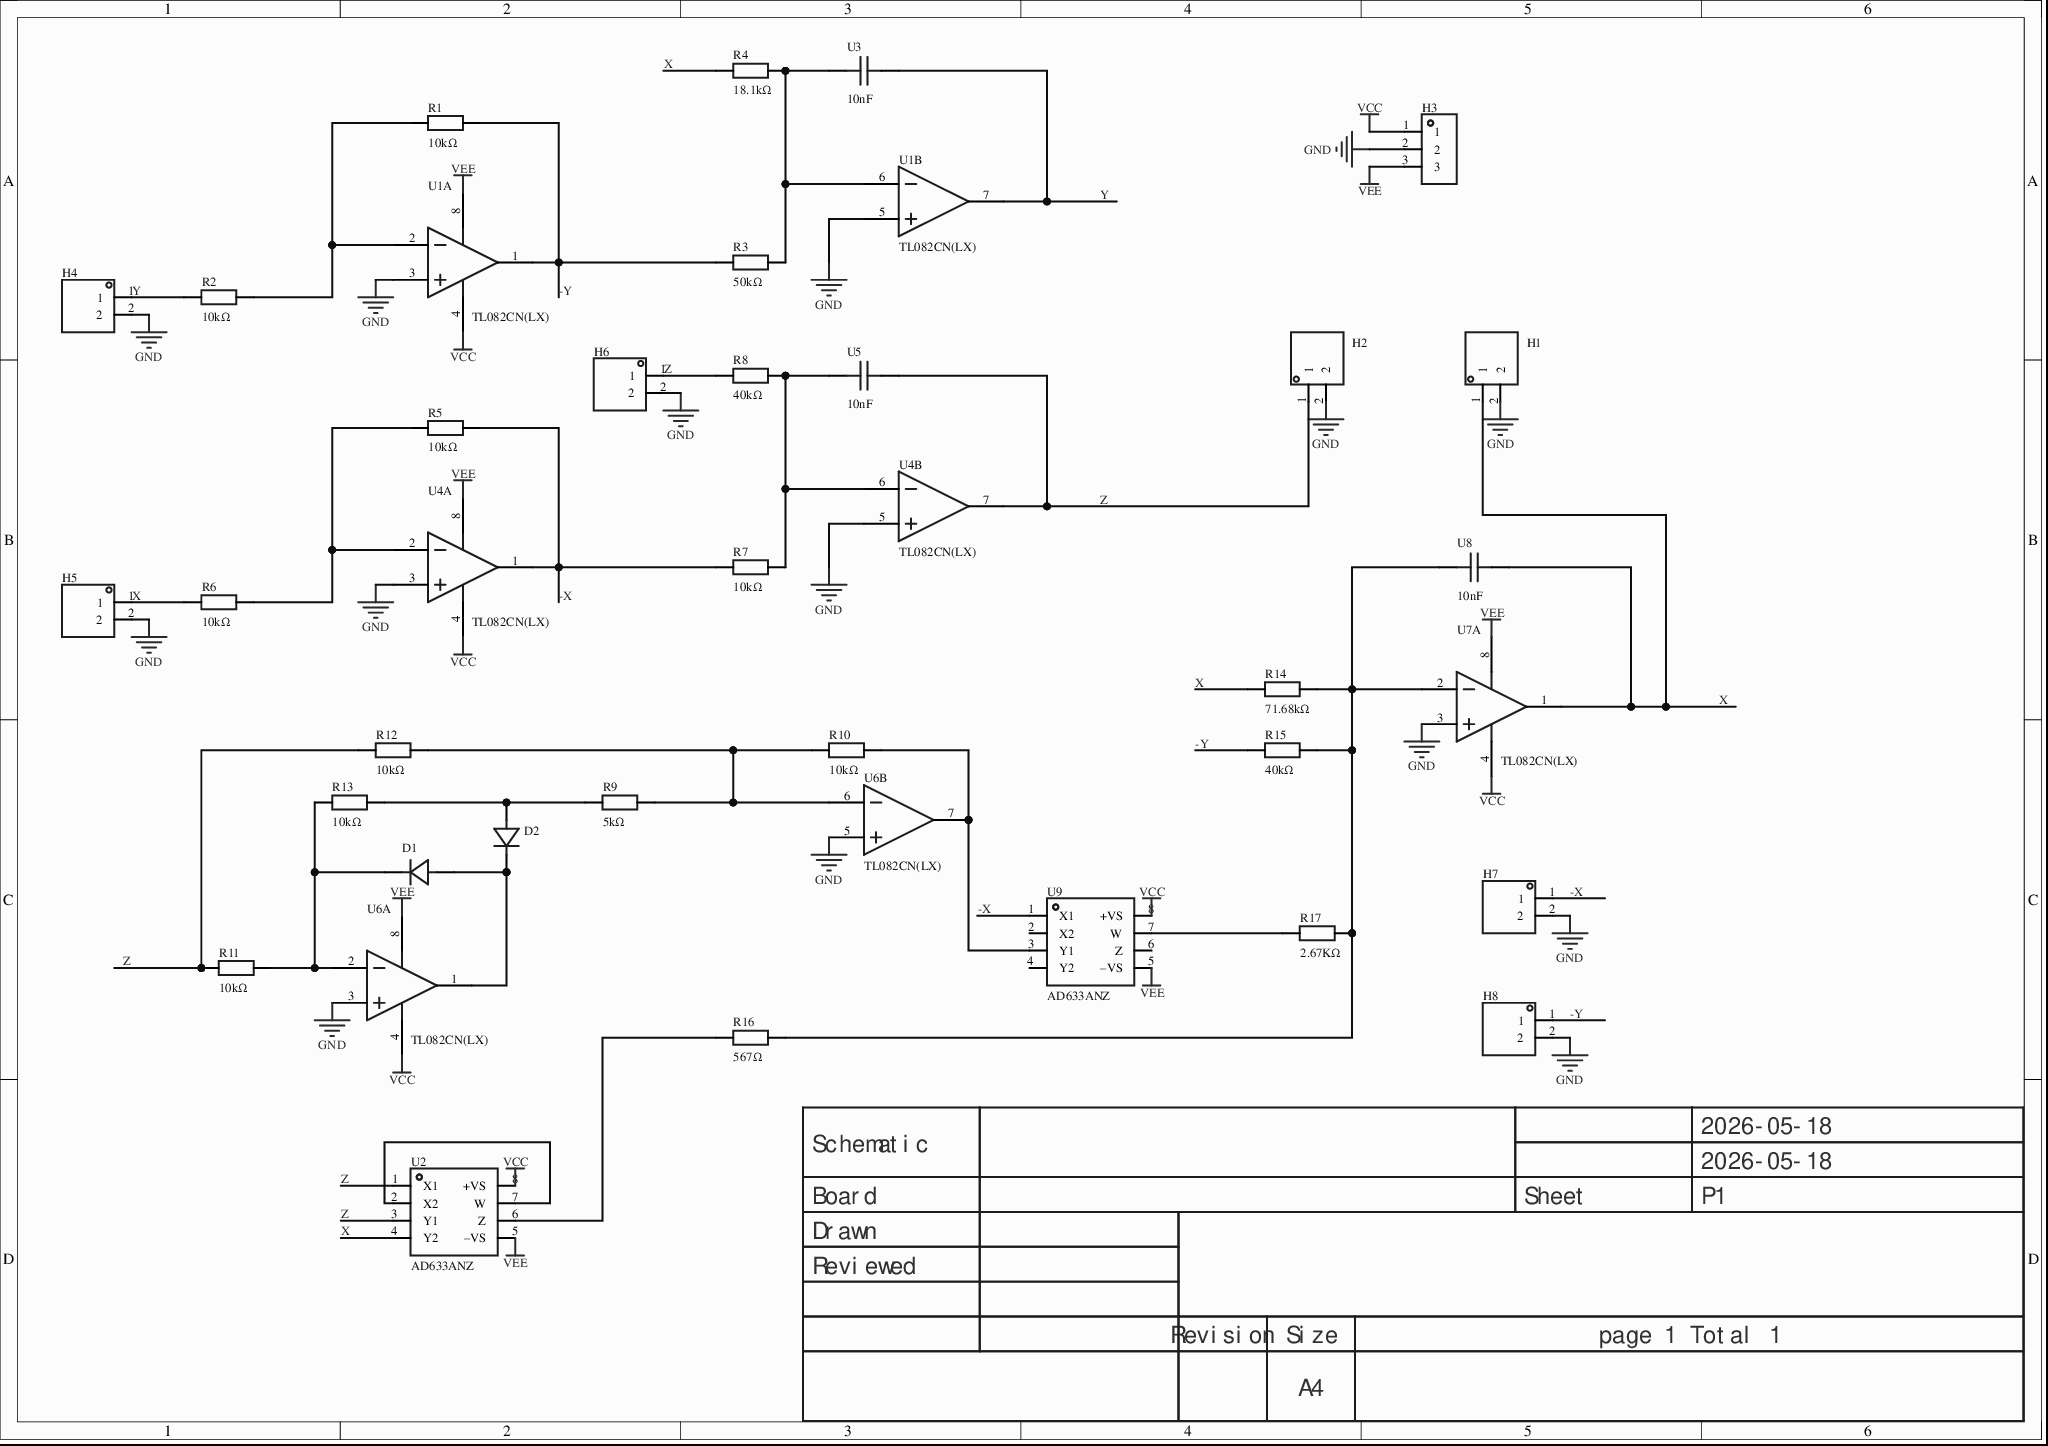
[diagram p0: MISC51419-3.schdoc]
# Altium project MISC51419-2.PrjPcb
1 sheet, 36 parts. Net scope: global (net labels, ports and power ports of the same name join across sheets).
Board file: MISC51419.pcbdoc

## Sheet MISC51419-3.schdoc
size 297 x 209 mm; Version: V1.0; @Project Name: MISC51419; @Update Date: 2026-05-18; @Create Date: 2026-05-18; @Board Name: MISC51419; @Create Time: 16:48:40; @Page Count: 1; @Page No: 1; @Schematic Name: MISC51419; @Update Time: 16:48:40; Size: A4

### Parts
D1  (no value)  [DO_1N4007]
D2  (no value)  [DO_1N4007]
H1  (no value)  [HDR-TH_2P-P2.54-V-M-1]
H2  (no value)  [HDR-TH_2P-P2.54-V-M-1]
H3  (no value)  [HDR-TH_3P-P2.54-V-M]
H4  (no value)  [HDR-TH_2P-P2.54-V-M-1]
H5  (no value)  [HDR-TH_2P-P2.54-V-M-1]
H6  (no value)  [HDR-TH_2P-P2.54-V-M-1]
H7  (no value)  [HDR-TH_2P-P2.54-V-M-1]
H8  (no value)  [HDR-TH_2P-P2.54-V-M-1]
R1  10kΩ  [Res_1/8W]
R2  10kΩ  [Res_1/8W]
R3  50kΩ  [Res_1/8W]
R4  18.1kΩ  [Res_1/8W]
R5  10kΩ  [Res_1/8W]
R6  10kΩ  [Res_1/8W]
R7  10kΩ  [Res_1/8W]
R8  40kΩ  [Res_1/8W]
R9  5kΩ  [Res_1/8W]
R10  10kΩ  [Res_1/8W]
R11  10kΩ  [Res_1/8W]
R12  10kΩ  [Res_1/8W]
R13  10kΩ  [Res_1/8W]
R14  71.68kΩ  [Res_1/8W]
R15  40kΩ  [Res_1/8W]
R16  567Ω  [Res_1/8W]
R17  2.67KΩ  [Res_1/8W]
U1  TL082CN(LX)  [PDIP-8_L9.6-W6.4-P2.54-LS7.6-BL]  (parts A,B of 2)
U2  AD633ANZ  [PDIP-8_L9.3-W6.4-P2.54-LS7.9-BL-1]
U3  10nF  [CAP-TH_L5.0-W2.5-P5.00-D1.0]
U4  TL082CN(LX)  [PDIP-8_L9.6-W6.4-P2.54-LS7.6-BL]  (parts A,B of 2)
U5  10nF  [CAP-TH_L5.0-W2.5-P5.00-D1.0]
U6  TL082CN(LX)  [PDIP-8_L9.6-W6.4-P2.54-LS7.6-BL]  (parts A,B of 2)
U7  TL082CN(LX)  [PDIP-8_L9.6-W6.4-P2.54-LS7.6-BL]  (part A of 2)
U8  10nF  [CAP-TH_L5.0-W2.5-P5.00-D1.0]
U9  AD633ANZ  [PDIP-8_L9.3-W6.4-P2.54-LS7.9-BL-1]

### Nets
GND: H1.2 H2.2 H3.2 H4.2 H5.2 H6.2 H7.2 H8.2 U1.3(IN1+) U1.5(IN2+) U4.3(IN1+) U4.5(IN2+) U6.3(IN1+) U6.5(IN2+) U7.3(IN1+)
VCC: H3.1 U1.4(VCC-) U2.8(+VS) U4.4(VCC-) U6.4(VCC-) U7.4(VCC-) U9.8(+VS)
VEE: H3.3 U1.8(VCC+) U2.5(–VS) U4.8(VCC+) U6.8(VCC+) U7.8(VCC+) U9.5(–VS)
-X: H7.1 R5.2 R7.1 U4.1(OUT1) U9.1(X1)
-Y: H8.1 R1.2 R3.1 R15.1 U1.1(OUT1)
X: H1.1 H5.1 R4.1 R6.1 R14.1 U2.4(Y2) U7.1(OUT1) U8.1
Y: H4.1 R2.1 U1.7(OUT2) U3.1
Z: H2.1 H6.1 R8.1 R11.1 R12.1 U2.1(X1) U2.3(Y1) U4.7(OUT2) U5.1
NetD1_1: D1.1(K) R11.2 R13.1 U6.2(IN1-)
NetD1_2: D1.2(A) D2.1(K) U6.1(OUT1)
NetD2_2: D2.2(A) R9.1 R13.2
NetR1_1: R1.1 R2.2 U1.2(IN1-)
NetR3_2: R3.2 R4.2 U1.6(IN2-) U3.2
NetR5_1: R5.1 R6.2 U4.2(IN1-)
NetR7_2: R7.2 R8.2 U4.6(IN2-) U5.2
NetR9_2: R9.2 R10.1 R12.2 U6.6(IN2-)
NetR10_2: R10.2 U6.7(OUT2) U9.3(Y1)
NetR14_2: R14.2 R15.2 R16.2 R17.2 U7.2(IN1-) U8.2
NetR16_1: R16.1 U2.6(Z)
NetR17_1: R17.1 U9.7(W)
NetU2_2: U2.2(X2) U2.7(W)

Not connected (* = marked no-connect by the designer): U9 2(X2) 4(Y2) 6(Z)

### Notes on the sheet
- 2026-05-18
- Schematic
- Board
- Sheet
- P1
- Drawn
- Reviewed
- Revision
- Size
- A4
- page 1 Total 1

### Library data of the parts
D1 D2 = D_1N4007A: AddInBom: yes; ModelId: 6de1e9b71a0d4751b4e9df530304c1a30819f05c4eef4c71ace90d822a990e87; ModelName: DO-41_D2.4-L4.7-P8.70; ModelTransform: 373.9,94.4,232.29,0,0,0,0,0,-140; Symbol: D_1N4007; Device: D_1N4007A; Supplier Footprint: DO-41; ConvertToPcb: yes; FootprintName: DO_1N4007
H1 H2 H4-H8 = HDR-M_2.54_1x2P: Symbol: 210S-1*2P L=11.6MMGold-plated black; ConvertToPcb: yes; ModelId: 79b2e9f2d70a4d68a1b7098f27c6d4c50819f05c4eef4c71ace90d822a990e87; ModelName: HDR-M-2.54_1x2; ModelTransform: 200,100,0,0,0,0,0,0,-118.11; Device: HDR-M_2.54_1x2P; AddInBom: yes; SupplierPart: C124375; Supplier Footprint: 插件; FootprintName: HDR-TH_2P-P2.54-V-M-1
H3 = HDR-M_2.54_1x3P: AddInBom: yes; ModelId: bb473b6d38ff42a99216a4fcdbdcc4cb0819f05c4eef4c71ace90d822a990e87; ModelName: HDR-TH_3P-P2.54-M-LI-1X3P; ModelTransform: 300.03877,100,0,0,0,0,0,0,-118.11; Symbol: HDR-M_2.54_1x3P; Device: HDR-M_2.54_1x3P; ConvertToPcb: yes; FootprintName: HDR-TH_3P-P2.54-V-M; SupplierPart: C2937625; Supplier Footprint: 插件
R1-R17 = Res_AXIAL-1/8W: Symbol: Resistor; ConvertToPcb: yes; ModelId: b2b5ae7ae4c642178fe0039925c86a3f0819f05c4eef4c71ace90d822a990e87; ModelName: RES-TH_BD1.8-L3.2-P7.20-D0.4; ModelTransform: 282.86,66.88,253.09,0,0,0,0,0,-191; Device: Res_AXIAL-1/8W; AddInBom: yes; Supplier Footprint: 轴向引线; FootprintName: Res_1/8W
  R1 R2 R5-R7 R10-R13: Value: 10kΩ
  R3: Value: 50kΩ
  R4: Value: 18.1kΩ
  R8 R15: Value: 40kΩ
  R9: Value: 5kΩ
  R14: Value: 71.68kΩ
  R16: Value: 567Ω
  R17: Value: 2.67KΩ
U1 U4 U6 U7 = TL082CN(LX): Amplifier count: 2; gain-bandwidth product (GBW): 1.3MHz; input offset voltage (Vos): 2mV; slew rate (SR): 14V/us; input bias current (Ib): 30pA;; Manufacturer: LX(灵星芯微); Relevance: []; AddInBom: yes; ModelId: 5dc2af053da0476fab11ee64b9a10a940819f05c4eef4c71ace90d822a990e87; ModelName: PDIP-8_L9.6-W6.4-P2.54-LS7.62-BL; ModelTransform: 377.952,309.842,0,0,0,0,0,0,-137.795; Number of Channels: 2; Maximum Power Supply Range (Vdd-Vss): 36V; Input Offset Voltage Drift(Vos TC): 18uV/℃; Input Offset Current(Ios): 5pA; Input Voltage Noise Density: 8nV/√Hz@1kHz; Common Mode Rejection Ratio(CMRR): 86dB; Quiescent Current: 1.2mA; Dual Supply: 5V~15V; -15V~-5V; Symbol: TL082CN(LX); Device: TL082CN(LX); LCSC Part Name: JFET输入双通道运放; SupplierPart: C49396714; ManufacturerPart: TL082CN(LX); Supplier Footprint: DIP-8; JLCPCB Part Class: Extended Part; Datasheet: https://example.com/datasheet/TL082CN(LX)/51919988.html; Supplier: LCSC; ConvertToPcb: yes; FootprintName: PDIP-8_L9.6-W6.4-P2.54-LS7.6-BL; Gain Bandwidth Product: 1.3MHz; Vos - Input Offset Voltage: 2mV; Slew Rate: 14V/us; Ib - Input Bias Current: 30pA; Operating Temperature: -40℃~+125℃
U2 U9 = AD633ANZ: Quadrant: four-quadrant; slew rate (SR): 20V/us; bandwidth: 1MHz;; Manufacturer: ADI(亚德诺); AddInBom: yes; ModelId: 28221afe73f64733a5f69edf09cc82000819f05c4eef4c71ace90d822a990e87; ModelTransform: 366.141,322.834,0,0,0,0,0,0,-118.11; Ib - Input Bias Current: 800nA; Maximum Power Supply Range (Vdd-Vss): 36V; Common Mode Rejection Ratio (CMRR): 80dB; Symbol: AD633ANZ; Device: AD633ANZ; LCSC Part Name: 低成本模拟乘法器; SupplierPart: C578355; ManufacturerPart: AD633ANZ; Supplier Footprint: PDIP-8; JLCPCB Part Class: Extended Part; Datasheet: https://example.com/datasheet/AD633ANZ/606132.html; Supplier: LCSC; ConvertToPcb: yes; FootprintName: PDIP-8_L9.3-W6.4-P2.54-LS7.9-BL-1; ModelName: PDIP-8_L9.3-W6.4-P2.54-LS7.9-BL-1; Quadrant: Four-quadrant; Slew Rate: 20V/us; Bandwidth: 1MHz; Operating Temperature: -40℃~+85℃
U3 U5 U8 = 100nF: Symbol: 100NF_C9900015256; AddInBom: yes; ModelId: 08e3d7481fc7486bb1b263873f51e1e10819f05c4eef4c71ace90d822a990e87; ModelName: CAP-TH_BD5.0-W2.5-P5.08; ModelTransform: 224.652,98.425,0,0,0,0,-0.005,0,-137.795; Device: 100nF; Manufacturer Part: 10nF; LCSC Part Name: 100nF; SupplierPart: C9900015256; Supplier Footprint: CAP-TH_L5.0-W2.5-P5.00-D1.0; JLCPCB Part Class: Extended Part; Supplier: LCSC; ConvertToPcb: yes; FootprintName: CAP-TH_L5.0-W2.5-P5.00-D1.0